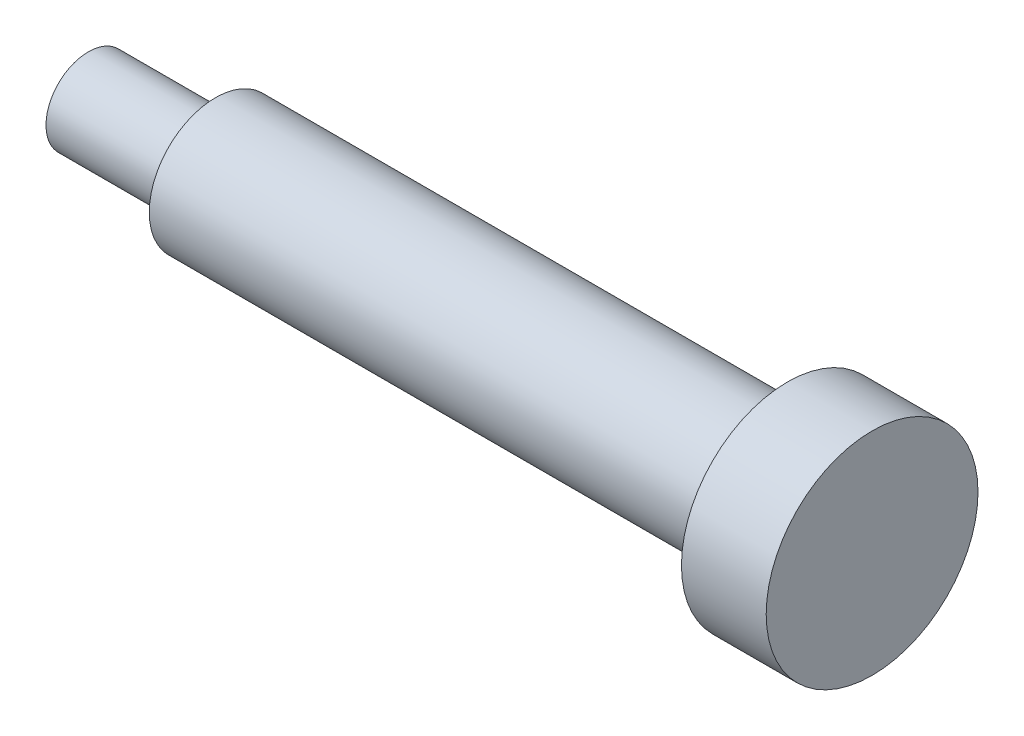
from build123d import *


with BuildPart() as part:
    # Sketch1 → Revolve1 (revolve)
    with BuildSketch(Plane.XY, mode=Mode.PRIVATE) as revolve1_sk:
        Polygon((-17.760797342, 0), (-17.760797342, -2), (-11.760797342, -2), (-11.760797342, -3.125), (15.239202658, -3.125), (15.239202658, -5), (19.239202658, -5), (19.239202658, 0), align=None)
    revolve(revolve1_sk.sketch.rotate(Axis((-26.641196013, 0, 0), (1, 0, 0)), 270), axis=Axis((-26.641196013, 0, 0), (1, 0, 0)))


solid = part.part
